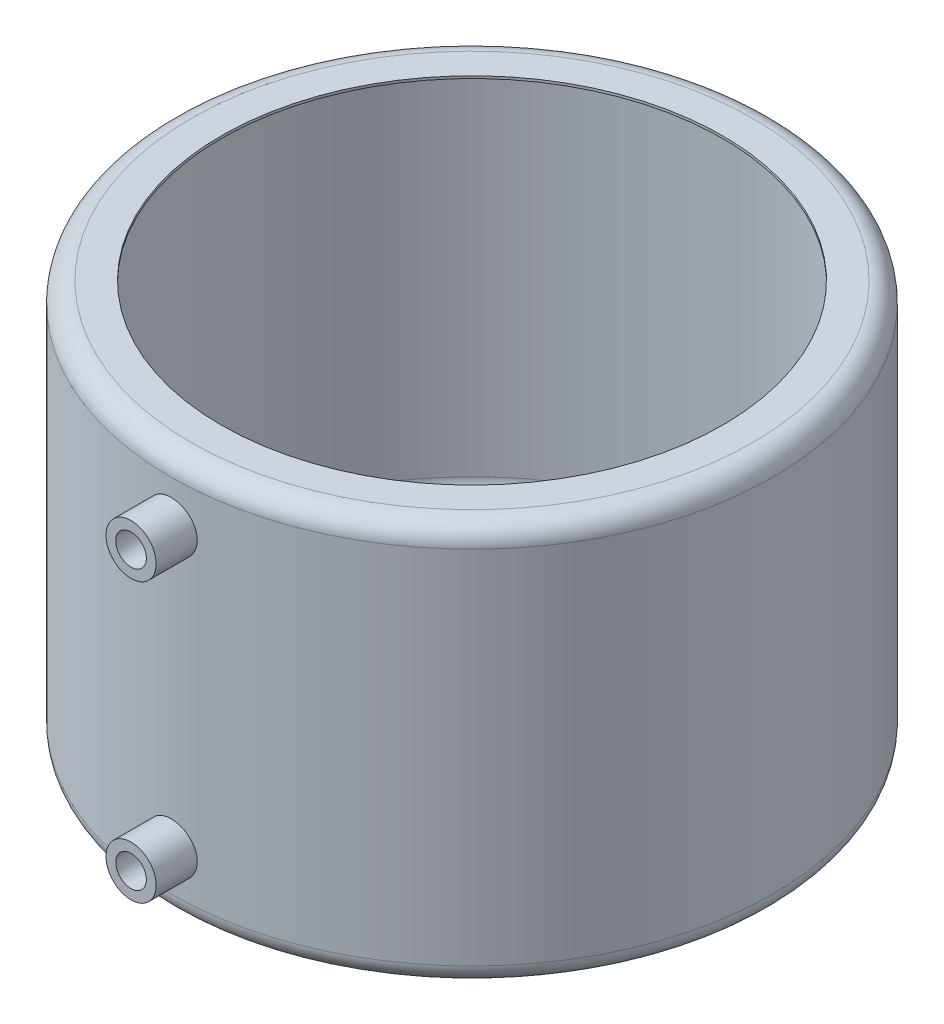
from build123d import *

# Parameters (mm, degrees)
SKETCH1_R                = 150
BOSS_EXTRUDE1_DEPTH      = 200
FILLET1_R                = 10
SKETCH2_R                = 125
CUT_EXTRUDE1_DEPTH       = 292.547594794
SHELL2_T                 = -1.2
BOSS_EXTRUDE2_REACH      = 408.079
BOSS_EXTRUDE2_END_RADIUS = 150
SKETCH5_R                = 12.5
G3_8_TAPPED_HOLE1_D      = 15.25
G3_8_TAPPED_HOLE1_DEPTH  = 37.33
G3_8_TAPPED_HOLE1_TIP    = 4.58156222


with BuildPart() as part:
    # Sketch1 → Boss-Extrude1 (new body)
    with BuildSketch(Plane(origin=(0, 0, 0), x_dir=(1, 0, 0), z_dir=(0, 1, 0))):
        with Locations(Location((0, 0, 0), (0, 0, 270))):
            Circle(SKETCH1_R)
    extrude(amount=BOSS_EXTRUDE1_DEPTH)

    # Fillet1
    fillet1_edges = [part.edges().sort_by_distance(p)[0] for p in [
        (0, 0, -150),
        (0, 200, -150),
    ]]
    fillet(fillet1_edges, radius=FILLET1_R)

    # Sketch2 → Cut-Extrude1 (cut, through all)
    with BuildSketch(Plane(origin=(0, 200, 0), x_dir=(1, 0, 0), z_dir=(0, 1, 0))):
        with Locations(Location((0, 0, 0), (0, 0, 270))):
            Circle(SKETCH2_R)
    extrude(amount=-CUT_EXTRUDE1_DEPTH, mode=Mode.SUBTRACT)

    # Shell2
    shell2_openings = [part.faces().sort_by_distance(p)[0] for p in [
        (0, 100, -125),
    ]]
    offset(amount=SHELL2_T, openings=shell2_openings, kind=Kind.INTERSECTION)

    # Boss-Extrude2: up to this cylinder (the profile starts outside it)
    boss_extrude2_end = Plane(origin=(0, 99.4, 0), z_dir=(0, -1, 0)) * Cylinder(BOSS_EXTRUDE2_END_RADIUS, 1255.958, mode=Mode.PRIVATE)
    # Sketch5 → Boss-Extrude2 (add, up to the surface)
    with BuildSketch(Plane.XY.offset(170), mode=Mode.PRIVATE) as boss_extrude2_sk1:
        with Locations((0, 30)):
            Circle(SKETCH5_R)
    boss_extrude2_tool1 = extrude(boss_extrude2_sk1.sketch, amount=-BOSS_EXTRUDE2_REACH, mode=Mode.PRIVATE) - boss_extrude2_end
    add(boss_extrude2_tool1.solids().sort_by_distance((0, 30, 170))[0])
    # Sketch5 → Boss-Extrude2 (add, up to the surface)
    with BuildSketch(Plane.XY.offset(170), mode=Mode.PRIVATE) as boss_extrude2_sk2:
        with Locations((0, 168.8)):
            Circle(SKETCH5_R)
    boss_extrude2_tool2 = extrude(boss_extrude2_sk2.sketch, amount=-BOSS_EXTRUDE2_REACH, mode=Mode.PRIVATE) - boss_extrude2_end
    add(boss_extrude2_tool2.solids().sort_by_distance((0, 168.8, 170))[0])

    # G3/8 Tapped Hole1
    with Locations(Plane(origin=(0, 30, 170), x_dir=(1, 0, 0), z_dir=(0, 0, 1))):
        with Locations((0, 0), (0, 138.8)):
            Hole(G3_8_TAPPED_HOLE1_D / 2, depth=G3_8_TAPPED_HOLE1_DEPTH)
            with Locations((0, 0, -(G3_8_TAPPED_HOLE1_DEPTH + G3_8_TAPPED_HOLE1_TIP / 2))):  # 118° drill point
                Cone(0, G3_8_TAPPED_HOLE1_D / 2, G3_8_TAPPED_HOLE1_TIP, mode=Mode.SUBTRACT)


solid = part.part
